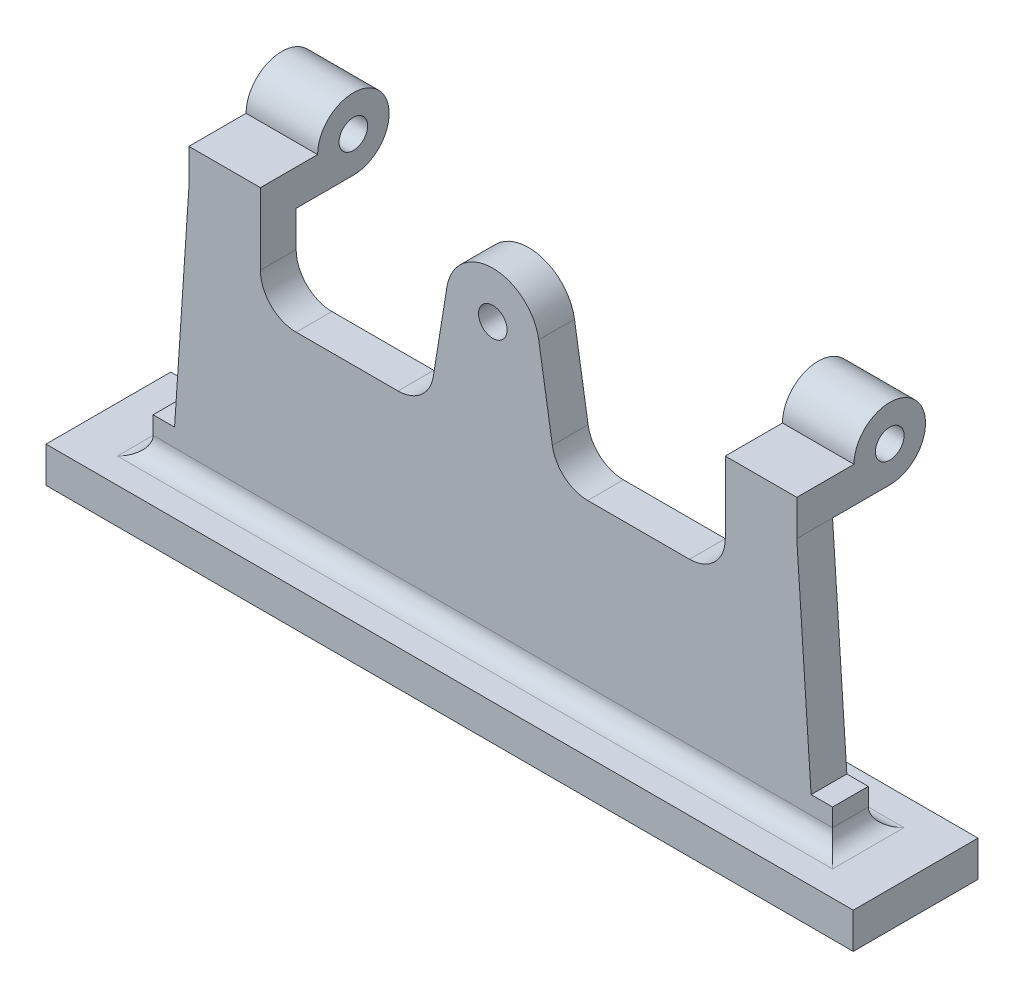
SolidWorks part; units mm, degrees
ref_plane "Front Plane" through (0, 0, 0) normal (0, 0, 1) x (1, 0, 0)
ref_plane "Top Plane" through (0, 0, 0) normal (0, 1, 0) x (1, 0, 0)
ref_plane "Right Plane" through (0, 0, 0) normal (1, 0, 0) x (0, 0, -1)
sketch "Sketch1" plane through (0, 0, 0) normal (0, 0, 1) x (1, 0, 0)
  line L0 (-85, -10) -> (-89, -70)
  line L1 (95, -80) -> (95, -70)
  line L2 (-95, -80) -> (95, -80)
  line L3 (95, -70) -> (89, -70)
  line L4 (12.8346, 2.0674) -> (16.6454, -21.5903)
  line L5 (0, 0) -> (0, -85) construction
  line L6 (-65, -10) -> (-65, -20)
  line L7 (-55, -30) -> (-26.5181, -30)
  line L8 (-12.8346, 2.0674) -> (-16.6454, -21.5903)
  line L9 (-65, -10) -> (-85, -10)
  line L10 (65, -10) -> (65, -20)
  line L11 (65, -10) -> (85, -10)
  line L12 (85, -10) -> (89, -70)
  line L13 (26.5181, -30) -> (55, -30)
  line L14 (-95, -80) -> (-95, -70)
  line L15 (-95, -70) -> (-89, -70)
  circle A0 centre (0, 0) radius 4
  arc A1 (12.8346, 2.0674) -> (-12.8346, 2.0674) centre (0, 0) ccw
  arc A2 (-65, -20) -> (-55, -30) centre (-55, -20) ccw
  arc A3 (-16.6454, -21.5903) -> (-26.5181, -30) centre (-26.5181, -20) cw
  arc A4 (16.6454, -21.5903) -> (26.5181, -30) centre (26.5181, -20) ccw
  arc A5 (65, -20) -> (55, -30) centre (55, -20) cw
  point P20 (-65, -30)
  point P24 (-18, -30)
  point P27 (18, -30)
  point P30 (65, -30)
  dimension "D2" = 95
  dimension "D3" = 80
  dimension "D6" = 26
  dimension "D10" = 8
  dimension "D13" = 10
  dimension "D16" = 10
  dimension "D4" = 6
  dimension "D5" = 190
  dimension "D7" = 6
  dimension "D8" = 10
  dimension "D9" = 10
  dimension "D11" = 50
  dimension "D12" = 36
  dimension "D14" = 170
  dimension "D15" = 130
extrude "Boss-Extrude1" add sketch "Sketch1" along normal blind 10
sketch "Sketch2" plane through (0, -80, 0) normal (0, -1, 0) x (-1, 0, 0)
  line L1 (-112.8717, 12.8044) -> (112.8717, 12.8044)
  line L2 (-112.8717, 12.8044) -> (-112.8717, -22.0819)
  line L3 (-112.8717, -22.0819) -> (112.8717, -22.0819)
  line L4 (112.8717, 12.8044) -> (112.8717, -22.0819)
  line L5 (-112.8717, 12.8044) -> (112.8717, -22.0819) construction
  line L6 (-112.8717, -22.0819) -> (112.8717, 12.8044) construction
  point P0 (0, -4.6388)
extrude "Boss-Extrude2" add sketch "Sketch2" along normal blind 10
sketch "Sketch3" plane through (-65, 0, 0) normal (1, 0, 0) x (0, 0, -1)
  line L0 (-10, -10) -> (0, -10) construction
  line L1 (0, -20) -> (0, -10) construction
  line L2 (6, 0) -> (-10, 0)
  line L3 (-10, 0) -> (-10, -10)
  line L4 (-10, -10) -> (16, -10)
  circle A0 centre (16, 0) radius 4
  arc A1 (16, -10) -> (6, 0) centre (16, 0) ccw
  dimension "D1" = 8
  dimension "D2" = 10
  dimension "D3" = 20
  dimension "D4" = 16
extrude "Boss-Extrude3" add sketch "Sketch3" against normal blind 20
mirror "Mirror1" about plane through (0, 0, 0) normal (1, 0, 0) of "Boss-Extrude3"
fillet "Fillet1" radius 5 4 edges at (0, -80, 10) (0, -80, 0) (-95, -80, 5) (95, -80, 5)
